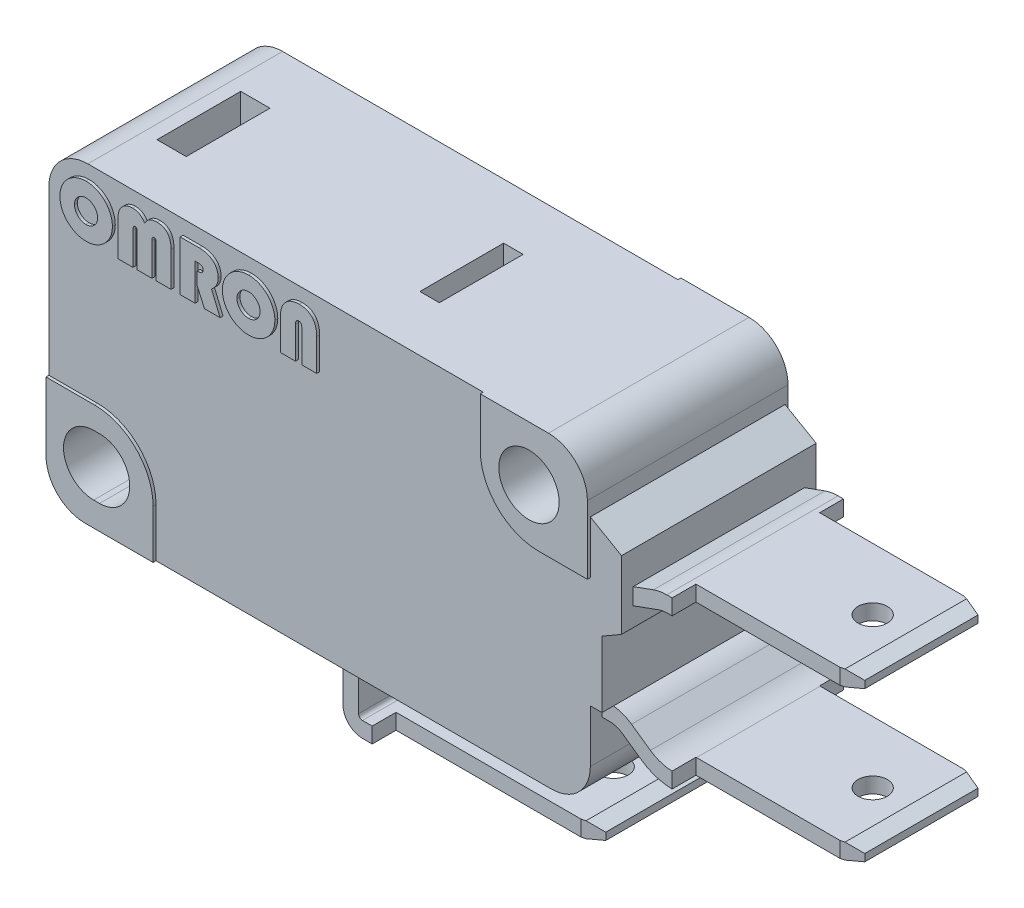
from build123d import *
from OCP.BRepFilletAPI import BRepFilletAPI_MakeChamfer

# Parameters (mm, degrees)
EXTRUDE_1_DEPTH     = 5
EXTRUDE_START       = 0.15
EXTRUDE_2_DEPTH     = 0.15
SKETCH_3_R          = 1.55
CUT_EXTRUDE_1_DEPTH = 21.237156421
CUT_EXTRUDE_2_DEPTH = 2.15
SKETCH_8_R          = 0.5
CUT_EXTRUDE_3_DEPTH = 3
EXTRUDE_3_DEPTH     = 4.4
SKETCH_10_R         = 0.75
SKETCH_10_W         = 8.4
SKETCH_10_H         = 1.225
CUT_EXTRUDE_4_DEPTH = 30.982870109
SKETCH_11_R         = 0.75
SKETCH_11_W         = 10.5
SKETCH_11_H         = 1.225
CUT_EXTRUDE_5_DEPTH = 1
CHAMFER_1_SIZE      = 0.8
CHAMFER_1_SIZE2     = 0.214359354
CHAMFER_2_SIZE      = 0.8
CHAMFER_2_SIZE2     = 0.214359354
CHAMFER_3_SIZE      = 1
CHAMFER_3_SIZE2     = 0.267949192
CHAMFER_4_SIZE      = 1
CHAMFER_4_SIZE2     = 0.267949192
EXTRUDE_6_DEPTH     = 0.15


with BuildPart() as part:
    # 草图1 → 凸台-拉伸1 (new, symmetric)
    with BuildSketch(Plane.XY):
        with BuildLine():
            Line((13.9, -3.25), (14.5, -3.25))
            Line((14.5, -3.25), (14.5, 0.1488893))
            Line((14.5, 0.1488893), (15.5, 0.726239569))
            Line((15.5, 0.726239569), (15.5, 4.226239569))
            Line((15.5, 4.226239569), (13.9, 5.15))
            Line((13.9, 5.15), (13.9, 5.95))
            ThreePointArc((13.9, 5.95), (13.314213562, 7.364213562), (11.9, 7.95))
            Line((11.9, 7.95), (-11.9, 7.95))
            ThreePointArc((-11.9, 7.95), (-13.314213562, 7.364213562), (-13.9, 5.95))
            Line((-13.9, 5.95), (-13.9, -5.95))
            ThreePointArc((-13.9, -5.95), (-13.314213562, -7.364213562), (-11.9, -7.95))
            Line((-11.9, -7.95), (11.9, -7.95))
            ThreePointArc((11.9, -7.95), (13.314213562, -7.364213562), (13.9, -5.95))
            Line((13.9, -5.95), (13.9, -3.25))
        make_face()
    extrude(amount=EXTRUDE_1_DEPTH, both=True)

    # 草图2 → 凸台-拉伸2 (add)
    with BuildSketch(Plane.XY.offset(5).offset(EXTRUDE_START)):
        with BuildLine():
            Line((-13.9, -2.45), (-11.4, -2.45))
            ThreePointArc((-11.4, -2.45), (-9.278679656, -3.328679656), (-8.4, -5.45))
            Line((-8.4, -5.45), (-8.4, -7.95))
            Line((-8.4, -7.95), (-11.9, -7.95))
            ThreePointArc((-11.9, -7.95), (-13.314213562, -7.364213562), (-13.9, -5.95))
            Line((-13.9, -5.95), (-13.9, -2.45))
        make_face()
        with BuildLine():
            Line((8.4, 7.95), (8.4, 5.45))
            ThreePointArc((8.4, 5.45), (9.278679656, 3.328679656), (11.4, 2.45))
            Line((11.4, 2.45), (13.9, 2.45))
            Line((13.9, 2.45), (13.9, 5.15))
            Line((13.9, 5.15), (13.9, 5.95))
            ThreePointArc((13.9, 5.95), (13.314213562, 7.364213562), (11.9, 7.95))
            Line((11.9, 7.95), (8.4, 7.95))
        make_face()
    extrude_2 = extrude(amount=-EXTRUDE_2_DEPTH)

    # 镜向1: 凸台-拉伸2 across plane
    add(extrude_2.mirror(Plane.XY))

    # 草图3 → 切除-拉伸1 (cut, through all)
    with BuildSketch(Plane.XY.offset(5.15)):
        with Locations((10.9, 5.15)):
            Circle(SKETCH_3_R)
        with BuildLine():
            Line((-11.45, -3.6), (-11.15, -3.6))
            ThreePointArc((-11.15, -3.6), (-9.6, -5.15), (-11.15, -6.7))
            Line((-11.15, -6.7), (-11.45, -6.7))
            ThreePointArc((-11.45, -6.7), (-13, -5.15), (-11.45, -3.6))
        make_face()
    extrude(amount=-CUT_EXTRUDE_1_DEPTH, mode=Mode.SUBTRACT)

    # 草图5 → 切除-拉伸2 (cut, symmetric)
    with BuildSketch(Plane.XY):
        with BuildLine():
            Line((-11.2, 7.95), (-9.7, 7.95))
            Line((-9.7, 7.95), (-9.7, 3.45))
            ThreePointArc((-9.7, 3.45), (-10.45, 2.7), (-11.2, 3.45))
            Line((-11.2, 3.45), (-11.2, 7.95))
        make_face()
        with BuildLine():
            Line((2.3, 7.95), (3.3, 7.95))
            Line((3.3, 7.95), (3.3, 6.05))
            ThreePointArc((3.3, 6.05), (2.8, 5.55), (2.3, 6.05))
            Line((2.3, 6.05), (2.3, 7.95))
        make_face()
    extrude(amount=CUT_EXTRUDE_2_DEPTH, both=True, mode=Mode.SUBTRACT)

    # 草图8 → 切除-拉伸3 (cut, symmetric)
    with BuildSketch(Plane.XY):
        with Locations((2.8, 6.05)):
            Circle(SKETCH_8_R)
    extrude(amount=CUT_EXTRUDE_3_DEPTH, both=True, mode=Mode.SUBTRACT)

    # 草图9 → 凸台-拉伸3 (add, symmetric)
    with BuildSketch(Plane.XY):
        with BuildLine():
            Line((0.6, -7.95), (0.6, -10.15))
            ThreePointArc((0.6, -10.15), (0.892893219, -10.857106781), (1.6, -11.15))
            Line((1.6, -11.15), (12.6, -11.15))
            Line((12.6, -11.15), (12.6, -10.35))
            Line((12.6, -10.35), (1.6, -10.35))
            ThreePointArc((1.6, -10.35), (1.458578644, -10.291421356), (1.4, -10.15))
            Line((1.4, -10.15), (1.4, -7.95))
            Line((1.4, -7.95), (0.6, -7.95))
        make_face()
        with BuildLine():
            Line((13.9, -3.25), (14.269402422, -3.25))
            ThreePointArc((14.269402422, -3.25), (14.870814021, -3.342566099), (15.416555295, -3.611695911))
            Line((15.416555295, -3.611695911), (16.382851914, -4.288304089))
            ThreePointArc((16.382851914, -4.288304089), (16.928593188, -4.557433901), (17.530004787, -4.65))
            Line((17.530004787, -4.65), (25.9, -4.65))
            Line((25.9, -4.65), (25.9, -5.45))
            Line((25.9, -5.45), (17.530004787, -5.45))
            ThreePointArc((17.530004787, -5.45), (16.688028549, -5.320407462), (15.923990765, -4.943625724))
            Line((15.923990765, -4.943625724), (14.957694146, -4.267017547))
            ThreePointArc((14.957694146, -4.267017547), (14.630249382, -4.105539659), (14.269402422, -4.05))
            Line((14.269402422, -4.05), (13.9, -4.05))
            Line((13.9, -4.05), (13.9, -3.25))
        make_face()
        with BuildLine():
            Line((15.5, 2.55), (16.542352384, 2.929385242))
            ThreePointArc((16.542352384, 2.929385242), (16.879096316, 3.019615506), (17.226392671, 3.05))
            Line((17.226392671, 3.05), (25.9, 3.05))
            Line((25.9, 3.05), (25.9, 2.25))
            Line((25.9, 2.25), (17.226392671, 2.25))
            ThreePointArc((17.226392671, 2.25), (17.018014858, 2.231769304), (16.815968499, 2.177631145))
            Line((16.815968499, 2.177631145), (15.5, 1.698657782))
            Line((15.5, 1.698657782), (15.5, 2.55))
        make_face()
    extrude(amount=EXTRUDE_3_DEPTH, both=True)

    # 草图10 → 切除-拉伸4 (cut, through all)
    with BuildSketch(Plane(origin=(0, 3.05, 0), x_dir=(1, 0, 0), z_dir=(0, 1, 0))):
        with Locations(Location((23.4, 0, 0), (0, 0, 180))):
            Circle(SKETCH_10_R)
        with Locations((21.7, 3.7875)):
            Rectangle(SKETCH_10_W, SKETCH_10_H)
        with Locations((21.7, -3.7875)):
            Rectangle(SKETCH_10_W, SKETCH_10_H)
    extrude(amount=-CUT_EXTRUDE_4_DEPTH, mode=Mode.SUBTRACT)

    # 草图11 → 切除-拉伸5 (cut)
    with BuildSketch(Plane.XZ.offset(11.15)):
        with Locations(Location((10.1, 0, 0), (0, 0, 270))):
            Circle(SKETCH_11_R)
        with Locations((7.35, 3.7875)):
            Rectangle(SKETCH_11_W, SKETCH_11_H)
        with Locations((7.35, -3.7875)):
            Rectangle(SKETCH_11_W, SKETCH_11_H)
    extrude(amount=-CUT_EXTRUDE_5_DEPTH, mode=Mode.SUBTRACT)

    # 倒角1: one chamfer whose edges measure the first distance from different faces: ONE call of the kernel's chamfer builder (chamfer() names one face for all edges)
    chamfer_1_edges_1 = [part.edges().sort_by_distance(p)[0] for p in [
        (25.9, 3.05, 0),
    ]]
    chamfer_1_side_1 = [part.faces().sort_by_distance(p)[0] for p in [
        (21.450909337, 3.05, 0),
    ]]
    chamfer_1_edges_2 = [part.edges().sort_by_distance(p)[0] for p in [
        (25.9, -4.65, 0),
    ]]
    chamfer_1_side_2 = [part.faces().sort_by_distance(p)[0] for p in [
        (21.657051792, -4.65, 0),
    ]]
    chamfer_1_edges_3 = [part.edges().sort_by_distance(p)[0] for p in [
        (12.6, -10.35, 0),
    ]]
    chamfer_1_side_3 = [part.faces().sort_by_distance(p)[0] for p in [
        (6.930716334, -10.35, 0),
    ]]
    chamfer_1 = BRepFilletAPI_MakeChamfer(part.part.solid().wrapped)
    for e in chamfer_1_edges_1:
        chamfer_1.Add(CHAMFER_1_SIZE, CHAMFER_1_SIZE2, e.wrapped, chamfer_1_side_1[0].wrapped)  # the first distance lies on this face
    for e in chamfer_1_edges_2:
        chamfer_1.Add(CHAMFER_1_SIZE, CHAMFER_1_SIZE2, e.wrapped, chamfer_1_side_2[0].wrapped)  # the first distance lies on this face
    for e in chamfer_1_edges_3:
        chamfer_1.Add(CHAMFER_1_SIZE, CHAMFER_1_SIZE2, e.wrapped, chamfer_1_side_3[0].wrapped)  # the first distance lies on this face
    add(Compound.cast(chamfer_1.Shape()), mode=Mode.REPLACE)

    # 倒角2: one chamfer whose edges measure the first distance from different faces: ONE call of the kernel's chamfer builder (chamfer() names one face for all edges)
    chamfer_2_edges_1 = [part.edges().sort_by_distance(p)[0] for p in [
        (25.9, 2.25, 0),
    ]]
    chamfer_2_side_1 = [part.faces().sort_by_distance(p)[0] for p in [
        (21.450909337, 2.25, 0),
    ]]
    chamfer_2_edges_2 = [part.edges().sort_by_distance(p)[0] for p in [
        (25.9, -5.45, 0),
    ]]
    chamfer_2_side_2 = [part.faces().sort_by_distance(p)[0] for p in [
        (21.657051792, -5.45, 0),
    ]]
    chamfer_2_edges_3 = [part.edges().sort_by_distance(p)[0] for p in [
        (12.6, -11.15, 0),
    ]]
    chamfer_2_side_3 = [part.faces().sort_by_distance(p)[0] for p in [
        (6.930716334, -11.15, 0),
    ]]
    chamfer_2 = BRepFilletAPI_MakeChamfer(part.part.solid().wrapped)
    for e in chamfer_2_edges_1:
        chamfer_2.Add(CHAMFER_2_SIZE, CHAMFER_2_SIZE2, e.wrapped, chamfer_2_side_1[0].wrapped)  # the first distance lies on this face
    for e in chamfer_2_edges_2:
        chamfer_2.Add(CHAMFER_2_SIZE, CHAMFER_2_SIZE2, e.wrapped, chamfer_2_side_2[0].wrapped)  # the first distance lies on this face
    for e in chamfer_2_edges_3:
        chamfer_2.Add(CHAMFER_2_SIZE, CHAMFER_2_SIZE2, e.wrapped, chamfer_2_side_3[0].wrapped)  # the first distance lies on this face
    add(Compound.cast(chamfer_2.Shape()), mode=Mode.REPLACE)

    # 倒角3: one chamfer whose edges measure the first distance from different faces: ONE call of the kernel's chamfer builder (chamfer() names one face for all edges)
    chamfer_3_edges_1 = [part.edges().sort_by_distance(p)[0] for p in [
        (25.9, -5.05, -3.175),
    ]]
    chamfer_3_side_1 = [part.faces().sort_by_distance(p)[0] for p in [
        (21.596996446, -5.049999764, -3.175),
    ]]
    chamfer_3_edges_2 = [part.edges().sort_by_distance(p)[0] for p in [
        (25.9, 2.65, -3.175),
    ]]
    chamfer_3_side_2 = [part.faces().sort_by_distance(p)[0] for p in [
        (21.596996847, 2.65, -3.175),
    ]]
    chamfer_3_edges_3 = [part.edges().sort_by_distance(p)[0] for p in [
        (12.6, -10.75, -3.175),
    ]]
    chamfer_3_side_3 = [part.faces().sort_by_distance(p)[0] for p in [
        (7.246144134, -10.75, -3.175),
    ]]
    chamfer_3 = BRepFilletAPI_MakeChamfer(part.part.solid().wrapped)
    for e in chamfer_3_edges_1:
        chamfer_3.Add(CHAMFER_3_SIZE, CHAMFER_3_SIZE2, e.wrapped, chamfer_3_side_1[0].wrapped)  # the first distance lies on this face
    for e in chamfer_3_edges_2:
        chamfer_3.Add(CHAMFER_3_SIZE, CHAMFER_3_SIZE2, e.wrapped, chamfer_3_side_2[0].wrapped)  # the first distance lies on this face
    for e in chamfer_3_edges_3:
        chamfer_3.Add(CHAMFER_3_SIZE, CHAMFER_3_SIZE2, e.wrapped, chamfer_3_side_3[0].wrapped)  # the first distance lies on this face
    add(Compound.cast(chamfer_3.Shape()), mode=Mode.REPLACE)

    # 倒角4: one chamfer whose edges measure the first distance from different faces: ONE call of the kernel's chamfer builder (chamfer() names one face for all edges)
    chamfer_4_edges_1 = [part.edges().sort_by_distance(p)[0] for p in [
        (25.9, -5.05, 3.175),
    ]]
    chamfer_4_side_1 = [part.faces().sort_by_distance(p)[0] for p in [
        (21.596996446, -5.049999764, 3.175),
    ]]
    chamfer_4_edges_2 = [part.edges().sort_by_distance(p)[0] for p in [
        (25.9, 2.65, 3.175),
    ]]
    chamfer_4_side_2 = [part.faces().sort_by_distance(p)[0] for p in [
        (21.596996847, 2.65, 3.175),
    ]]
    chamfer_4_edges_3 = [part.edges().sort_by_distance(p)[0] for p in [
        (12.6, -10.75, 3.175),
    ]]
    chamfer_4_side_3 = [part.faces().sort_by_distance(p)[0] for p in [
        (7.246144134, -10.75, 3.175),
    ]]
    chamfer_4 = BRepFilletAPI_MakeChamfer(part.part.solid().wrapped)
    for e in chamfer_4_edges_1:
        chamfer_4.Add(CHAMFER_4_SIZE, CHAMFER_4_SIZE2, e.wrapped, chamfer_4_side_1[0].wrapped)  # the first distance lies on this face
    for e in chamfer_4_edges_2:
        chamfer_4.Add(CHAMFER_4_SIZE, CHAMFER_4_SIZE2, e.wrapped, chamfer_4_side_2[0].wrapped)  # the first distance lies on this face
    for e in chamfer_4_edges_3:
        chamfer_4.Add(CHAMFER_4_SIZE, CHAMFER_4_SIZE2, e.wrapped, chamfer_4_side_3[0].wrapped)  # the first distance lies on this face
    add(Compound.cast(chamfer_4.Shape()), mode=Mode.REPLACE)

    # 草图12 → 凸台-拉伸6 (add)
    # profile 1 of 5: a face of its own
    with BuildSketch(Plane.XY.offset(5)):
        with BuildLine():
            add(Edge.make_bspline(
                [(-11.839991798, 7.284851975), (-11.810073224, 7.284327276), (-11.750675759, 7.283285589), (-11.662283846, 7.274595125), (-11.575549668, 7.260812561), (-11.490214484, 7.241324627), (-11.406864613, 7.215353494), (-11.324502331, 7.185023297), (-11.244436385, 7.1478037), (-11.165899619, 7.106345186), (-11.090511472, 7.059561807), (-11.018297745, 7.008864953), (-10.950378811, 6.95373237), (-10.886701297, 6.894389736), (-10.826790936, 6.831277485), (-10.771135463, 6.763895002), (-10.719655155, 6.692187959), (-10.672730505, 6.616922671), (-10.630327479, 6.539049624), (-10.593456274, 6.45921368), (-10.562226952, 6.377688868), (-10.536396609, 6.294753684), (-10.517163106, 6.210101031), (-10.502331332, 6.124247216), (-10.493964618, 6.036701875), (-10.492870367, 5.977867341), (-10.492320887, 5.948323445)],
                knots=[0, 0, 0, 0, 1.021661308, 2.028308306, 3.030389079, 4.019702427, 5.014833943, 6.01032923, 7.015036116, 8.027997564, 9.041872037, 10.04316966, 11.039694905, 12.027034081, 13.014087999, 14.009724715, 15.009534675, 16.026756487, 17.037133186, 18.036077674, 19.027888702, 20.016958036, 21.000091493, 21.990684927, 22.991017831, 24, 24, 24, 24], degree=3))
            add(Edge.make_bspline(
                [(-10.492320887, 5.948323445), (-10.492870761, 5.918779673), (-10.493965794, 5.859945386), (-10.502326694, 5.772398208), (-10.517180262, 5.686551281), (-10.536293747, 5.602046231), (-10.562352659, 5.519370522), (-10.593412015, 5.437969296), (-10.630511869, 5.358069672), (-10.672390966, 5.279897616), (-10.719854097, 5.204951969), (-10.771116293, 5.133302457), (-10.826761684, 5.065889776), (-10.886923526, 5.002874533), (-10.949968186, 4.942805024), (-11.018701336, 4.888496279), (-11.090282184, 4.836947876), (-11.165961989, 4.790412657), (-11.244257983, 4.748631429), (-11.324795915, 4.71252768), (-11.406606692, 4.680921455), (-11.490346315, 4.656110733), (-11.575528182, 4.636325447), (-11.662289633, 4.62262666), (-11.750674285, 4.613913889), (-11.81007273, 4.612875215), (-11.839991798, 4.612352033)],
                knots=[0, 0, 0, 0, 1.009153083, 2.009655437, 3.000416671, 3.983716664, 4.96689387, 5.958872904, 6.957986607, 7.974114181, 8.986134409, 9.986113729, 10.9819191, 11.969140218, 12.960977253, 13.95368625, 14.958823603, 15.972869819, 16.986002856, 17.988253375, 18.986157985, 19.979616663, 20.969097594, 21.971348113, 22.978165629, 24, 24, 24, 24], degree=3))
            add(Edge.make_bspline(
                [(-11.839991798, 4.612352033), (-11.869910881, 4.61287518), (-11.929309358, 4.613913786), (-12.017693781, 4.622627065), (-12.104456089, 4.636323945), (-12.189634791, 4.656116272), (-12.273386259, 4.68090064), (-12.355310552, 4.712667156), (-12.436166343, 4.748477792), (-12.514569817, 4.790432512), (-12.590260895, 4.836942604), (-12.661838761, 4.888497665), (-12.730572677, 4.942804661), (-12.793617211, 5.002874606), (-12.853778795, 5.065889843), (-12.909425354, 5.133302108), (-12.960683095, 5.204953308), (-13.008163097, 5.279892539), (-13.049979178, 5.358088563), (-13.087282054, 5.437840502), (-13.117475547, 5.519500144), (-13.143736666, 5.602028431), (-13.162790692, 5.686556088), (-13.177660321, 5.772396908), (-13.186016936, 5.859945716), (-13.187112546, 5.918779783), (-13.187662709, 5.948323445)],
                knots=[0, 0, 0, 0, 1.021684044, 2.028353444, 3.030456519, 4.019791883, 5.013104409, 6.010862213, 7.018749798, 8.031733789, 9.045630825, 10.050620308, 11.043183264, 12.034874386, 13.02195027, 14.017609144, 15.017441353, 16.029312699, 17.045290786, 18.044257506, 19.033836829, 20.016869396, 21.000024732, 21.990640211, 22.990995377, 24, 24, 24, 24], degree=3))
            add(Edge.make_bspline(
                [(-13.187662709, 5.948323445), (-13.187112939, 5.977867231), (-13.186018112, 6.036701546), (-13.177655681, 6.124248515), (-13.162807851, 6.210096225), (-13.143633913, 6.294771527), (-13.117599886, 6.377558735), (-13.087237778, 6.45934248), (-13.050163925, 6.53903087), (-13.007823594, 6.61692776), (-12.960882032, 6.692186619), (-12.909406184, 6.76389535), (-12.853749543, 6.831277418), (-12.793839438, 6.894389662), (-12.730162056, 6.953732737), (-12.662242332, 7.008863545), (-12.590031666, 7.059567124), (-12.514631925, 7.106325077), (-12.435989008, 7.147957464), (-12.355603598, 7.184885152), (-12.273128647, 7.215374716), (-12.189766541, 7.241318981), (-12.104434625, 7.260814091), (-12.017699562, 7.274594713), (-11.929307885, 7.283285694), (-11.869910388, 7.284327311), (-11.839991798, 7.284851975)],
                knots=[0, 0, 0, 0, 1.00883439, 2.009020783, 2.999469132, 3.982458596, 4.971383068, 5.960795436, 6.959593616, 7.969822333, 8.98689516, 9.986558684, 10.982049577, 11.968958928, 12.956153496, 13.952532787, 14.953683757, 15.967409735, 16.980222822, 17.99055106, 18.985900543, 19.98088631, 20.97005476, 21.971988766, 22.978488327, 24, 24, 24, 24], degree=3))
        make_face()
        with BuildLine():
            add(Edge.make_bspline(
                [(-11.843891631, 5.35944864), (-11.823816343, 5.360043883), (-11.784071756, 5.361222332), (-11.725518417, 5.368774544), (-11.669474516, 5.383075873), (-11.615765049, 5.40207715), (-11.563924484, 5.425952438), (-11.515020492, 5.456468843), (-11.467842494, 5.491658767), (-11.423744945, 5.532083862), (-11.383525093, 5.576133779), (-11.347943814, 5.622839772), (-11.317796046, 5.671604795), (-11.293723612, 5.722956508), (-11.274747747, 5.77613103), (-11.260505509, 5.831437776), (-11.252853781, 5.889239011), (-11.25170169, 5.928432438), (-11.251116993, 5.948323445)],
                knots=[0, 0, 0, 0, 1.037369248, 2.053759453, 3.042788757, 4.01997185, 4.994371679, 5.985028633, 6.992502963, 8.031645644, 9.070788326, 10.070603235, 11.061260189, 12.026976158, 12.995120048, 13.974843604, 14.972215384, 16, 16, 16, 16], degree=3))
            add(Edge.make_bspline(
                [(-11.251116993, 5.948323445), (-11.251614097, 5.968229317), (-11.252594243, 6.007477938), (-11.261533408, 6.065225549), (-11.274408552, 6.121260415), (-11.294245, 6.174676566), (-11.31895887, 6.226044923), (-11.349348226, 6.275199911), (-11.384816155, 6.322702568), (-11.426187787, 6.366584455), (-11.470069664, 6.40795582), (-11.5175721, 6.44342477), (-11.566727945, 6.473810454), (-11.618093157, 6.498537721), (-11.671351474, 6.518260907), (-11.727155856, 6.53131824), (-11.784740379, 6.540164447), (-11.82398685, 6.541153553), (-11.843891631, 6.541655202)],
                knots=[0, 0, 0, 0, 1.025725638, 2.022434234, 3.007203552, 3.985667517, 4.953578649, 5.942251004, 6.961114924, 8.0046544, 9.048193875, 10.067057795, 11.05573015, 12.023641282, 13.002105247, 13.977565766, 14.974274362, 16, 16, 16, 16], degree=3))
            add(Edge.make_bspline(
                [(-11.843891631, 6.541655202), (-11.86379772, 6.541158584), (-11.903046768, 6.540179396), (-11.960791258, 6.53123323), (-12.016837752, 6.518384167), (-12.070368114, 6.498392746), (-12.122038945, 6.473945443), (-12.17128493, 6.443603613), (-12.218333824, 6.407586087), (-12.262688797, 6.36678028), (-12.304114535, 6.322854765), (-12.338933997, 6.275020764), (-12.369411721, 6.22606679), (-12.394087265, 6.17467069), (-12.413934029, 6.121262007), (-12.426806378, 6.065225118), (-12.435746293, 6.00747805), (-12.436726336, 5.968229355), (-12.437223388, 5.948323445)],
                knots=[0, 0, 0, 0, 1.024980994, 2.020966011, 3.005020418, 3.982774049, 4.958606057, 5.946560666, 6.957057065, 8.006883537, 9.049665437, 10.062062882, 11.050017492, 12.017225951, 12.994979582, 13.979033989, 14.975019006, 16, 16, 16, 16], degree=3))
            add(Edge.make_bspline(
                [(-12.437223388, 5.948323445), (-12.436638692, 5.928432438), (-12.435486601, 5.889239011), (-12.427834872, 5.831437776), (-12.413592635, 5.776131028), (-12.394616766, 5.722956515), (-12.370544348, 5.671604768), (-12.34039652, 5.622839874), (-12.304815469, 5.576133388), (-12.264594735, 5.532085384), (-12.220500468, 5.491653169), (-12.173310652, 5.456488886), (-12.124306511, 5.425789862), (-12.072138947, 5.402215876), (-12.018319076, 5.383053554), (-11.962261993, 5.368780707), (-11.903712244, 5.361220736), (-11.863967167, 5.360043348), (-11.843891631, 5.35944864)],
                knots=[0, 0, 0, 0, 1.027226011, 2.024055714, 3.003246787, 3.970864486, 4.936055584, 5.926174111, 6.925445617, 7.964023519, 9.002601422, 10.009528185, 10.999646713, 11.982213023, 12.958865012, 13.947356774, 14.963194567, 16, 16, 16, 16], degree=3))
        make_face(mode=Mode.SUBTRACT)
    # profile 2 of 5: a face of its own
    with BuildSketch(Plane.XY.offset(5)):
        with BuildLine():
            Line((-10.199833401, 4.654693079), (-10.199833401, 6.507113822))
            add(Edge.make_bspline(
                [(-10.199833401, 6.507113822), (-10.199238422, 6.535004889), (-10.19807221, 6.589673842), (-10.187517826, 6.669762946), (-10.171836884, 6.746165648), (-10.148794096, 6.818580558), (-10.119173777, 6.886932172), (-10.082787005, 6.951382185), (-10.039586228, 7.011665795), (-9.990645064, 7.067944512), (-9.936573418, 7.118795455), (-9.87813828, 7.16326071), (-9.815943005, 7.20080454), (-9.749816998, 7.231590689), (-9.679773702, 7.255578142), (-9.606084879, 7.272856225), (-9.528603921, 7.283007754), (-9.475794682, 7.28422871), (-9.448836962, 7.284851975)],
                knots=[0, 0, 0, 0, 1.102663291, 2.161317456, 3.189909821, 4.184149151, 5.161173166, 6.13146464, 7.105723695, 8.089680947, 9.077004599, 10.036307647, 10.9886396, 11.944900811, 12.915859305, 13.911806509, 14.934032427, 16, 16, 16, 16], degree=3))
            add(Edge.make_bspline(
                [(-9.448836962, 7.284851975), (-9.416618779, 7.283914898), (-9.353734749, 7.282085893), (-9.262632689, 7.263903062), (-9.17690412, 7.236352199), (-9.097031368, 7.196398955), (-9.023432705, 7.144351472), (-8.95571787, 7.081214142), (-8.893172709, 7.007369039), (-8.858343365, 6.951437988), (-8.840462991, 6.922724612)],
                knots=[0, 0, 0, 0, 1.037369451, 2.024756404, 2.982649248, 3.933049122, 4.891334709, 5.878358653, 6.910810976, 8, 8, 8, 8], degree=3))
            add(Edge.make_bspline(
                [(-8.840462991, 6.922724612), (-8.821065782, 6.952539658), (-8.783628759, 7.010083327), (-8.718469493, 7.086078868), (-8.648561866, 7.148949243), (-8.573554847, 7.200173438), (-8.491188448, 7.238270959), (-8.400897054, 7.265759021), (-8.301737773, 7.281758752), (-8.232705063, 7.283797312), (-8.196990522, 7.284851975)],
                knots=[0, 0, 0, 0, 1.097134874, 2.117493542, 3.079635451, 3.992275589, 4.910372732, 5.869641242, 6.897844434, 8, 8, 8, 8], degree=3))
            add(Edge.make_bspline(
                [(-8.196990522, 7.284851975), (-8.168919377, 7.284235317), (-8.114259941, 7.283034574), (-8.034723952, 7.272990171), (-7.960396511, 7.255842073), (-7.891149015, 7.231620814), (-7.82679159, 7.201211791), (-7.767775075, 7.16322197), (-7.713165151, 7.119317205), (-7.664862413, 7.067387177), (-7.621020871, 7.010024136), (-7.583693985, 6.94584389), (-7.552063447, 6.875956796), (-7.525558304, 6.800166437), (-7.505900306, 6.717975024), (-7.491636394, 6.629893059), (-7.482389586, 6.5357228), (-7.48153416, 6.470923836), (-7.481092581, 6.437473945)],
                knots=[0, 0, 0, 0, 1.066598017, 2.076853064, 3.040727948, 3.960382046, 4.860103194, 5.73921303, 6.622167718, 7.515861307, 8.427763883, 9.361048407, 10.330694431, 11.33961724, 12.407802041, 13.537962884, 14.72907115, 16, 16, 16, 16], degree=3))
            Line((-7.481092581, 6.437473945), (-7.481092581, 4.654693079))
            Line((-7.481092581, 4.654693079), (-8.247131234, 4.654693079))
            Line((-8.247131234, 4.654693079), (-8.247131234, 6.326050141))
            add(Edge.make_bspline(
                [(-8.247131234, 6.326050141), (-8.247250471, 6.343329859), (-8.247470091, 6.375157126), (-8.251296244, 6.418738159), (-8.257206105, 6.454219499), (-8.264998956, 6.482392649), (-8.277012757, 6.504351653), (-8.294788532, 6.519549951), (-8.317622192, 6.52885694), (-8.334502661, 6.529573324), (-8.343512825, 6.529955702)],
                knots=[0, 0, 0, 0, 1.623684708, 2.990641638, 4.106939268, 5.001409125, 5.728884434, 6.421825748, 7.157629609, 8, 8, 8, 8], degree=3))
            add(Edge.make_bspline(
                [(-8.343512825, 6.529955702), (-8.352716482, 6.529588781), (-8.370386749, 6.528884323), (-8.394628553, 6.518737073), (-8.414840674, 6.503056471), (-8.431504982, 6.481464613), (-8.444001864, 6.453803192), (-8.452598283, 6.420257693), (-8.458221505, 6.38102107), (-8.458622368, 6.352814337), (-8.458836462, 6.33774964)],
                knots=[0, 0, 0, 0, 0.870208494, 1.670728877, 2.451709394, 3.282275218, 4.238613916, 5.318652993, 6.56794201, 8, 8, 8, 8], degree=3))
            Line((-8.458836462, 6.33774964), (-8.458836462, 4.654693079))
            Line((-8.458836462, 4.654693079), (-9.221532401, 4.654693079))
            Line((-9.221532401, 4.654693079), (-9.221532401, 6.326050141))
            add(Edge.make_bspline(
                [(-9.221532401, 6.326050141), (-9.221651038, 6.342773209), (-9.221870255, 6.373674252), (-9.225758459, 6.416320921), (-9.231692732, 6.451595646), (-9.239444844, 6.480389514), (-9.251826208, 6.50316279), (-9.270403356, 6.519100776), (-9.294361722, 6.529036497), (-9.312235735, 6.52963499), (-9.321813825, 6.529955702)],
                knots=[0, 0, 0, 0, 1.554968012, 2.873284574, 3.977956704, 4.879642019, 5.638089054, 6.348181832, 7.114845454, 8, 8, 8, 8], degree=3))
            add(Edge.make_bspline(
                [(-9.321813825, 6.529955702), (-9.330655607, 6.529367056), (-9.347607888, 6.528238448), (-9.371053683, 6.51789693), (-9.39131704, 6.5019435), (-9.406903874, 6.478412297), (-9.419084005, 6.449115876), (-9.426774177, 6.41344544), (-9.432702268, 6.371929501), (-9.433050946, 6.342048476), (-9.433237629, 6.326050141)],
                knots=[0, 0, 0, 0, 0.812646849, 1.558081647, 2.326829032, 3.164255741, 4.132651413, 5.243379863, 6.524102441, 8, 8, 8, 8], degree=3))
            Line((-9.433237629, 6.326050141), (-9.433237629, 4.654693079))
            Line((-9.433237629, 4.654693079), (-10.199833401, 4.654693079))
        make_face()
    # profile 3 of 5: a face of its own
    with BuildSketch(Plane.XY.offset(5)):
        with BuildLine():
            Line((-6.245402593, 6.529955702), (-6.245402593, 4.654693079))
            Line((-6.245402593, 4.654693079), (-7.008098532, 4.654693079))
            Line((-7.008098532, 4.654693079), (-7.008098532, 7.223011764))
            Line((-7.008098532, 7.223011764), (-6.029797532, 7.223011764))
            add(Edge.make_bspline(
                [(-6.029797532, 7.223011764), (-5.993184145, 7.222261302), (-5.921824432, 7.220798648), (-5.817875425, 7.209493673), (-5.719861379, 7.191188398), (-5.627557429, 7.165848091), (-5.541374844, 7.132277188), (-5.461170845, 7.091327811), (-5.386490918, 7.043443953), (-5.318923955, 6.987632711), (-5.257847466, 6.926389158), (-5.205057527, 6.85978581), (-5.159014627, 6.789391044), (-5.123176891, 6.713564327), (-5.094335602, 6.633770947), (-5.07386895, 6.549368718), (-5.061294341, 6.460324949), (-5.059971173, 6.399446499), (-5.059296198, 6.368391186)],
                knots=[0, 0, 0, 0, 1.205518528, 2.349562907, 3.438641392, 4.486182617, 5.496929055, 6.478808746, 7.447400395, 8.412103695, 9.359141492, 10.290349245, 11.20639267, 12.122701433, 13.045416251, 13.996178639, 14.977810715, 16, 16, 16, 16], degree=3))
            add(Edge.make_bspline(
                [(-5.059296198, 6.368391186), (-5.06044182, 6.336208837), (-5.06269386, 6.272945407), (-5.078292373, 6.179910158), (-5.106102258, 6.091663845), (-5.143493353, 6.006998913), (-5.192703932, 5.927215725), (-5.251602615, 5.850591662), (-5.322007368, 5.77870919), (-5.375282601, 5.735722554), (-5.402481515, 5.713776337)],
                knots=[0, 0, 0, 0, 1.006052783, 1.977678795, 2.938069743, 3.891839897, 4.863622002, 5.861128799, 6.908029685, 8, 8, 8, 8], degree=3))
            Line((-5.402481515, 5.713776337), (-4.959571894, 4.654693079))
            Line((-4.959571894, 4.654693079), (-5.76405176, 4.654693079))
            Line((-5.76405176, 4.654693079), (-6.133978789, 5.482571944))
            Line((-6.133978789, 5.482571944), (-6.133978789, 6.141086626))
            Line((-6.133978789, 6.141086626), (-6.072138578, 6.141086626))
            add(Edge.make_bspline(
                [(-6.072138578, 6.141086626), (-6.053152367, 6.141686707), (-6.017511835, 6.142813168), (-5.967592011, 6.152125962), (-5.924910508, 6.16797953), (-5.889714063, 6.191384539), (-5.862265859, 6.22159601), (-5.842876301, 6.258556678), (-5.831879689, 6.301844162), (-5.830511666, 6.332670832), (-5.829791804, 6.348892021)],
                knots=[0, 0, 0, 0, 1.246893405, 2.340643143, 3.321932138, 4.218857632, 5.091461181, 5.975846322, 6.934877491, 8, 8, 8, 8], degree=3))
            add(Edge.make_bspline(
                [(-5.829791804, 6.348892021), (-5.830614098, 6.363101335), (-5.832188454, 6.39030633), (-5.845229387, 6.428760947), (-5.86854753, 6.460695828), (-5.90018688, 6.487148737), (-5.941041681, 6.50609175), (-5.989723495, 6.520788519), (-6.047386319, 6.528519842), (-6.088647499, 6.529457364), (-6.11057979, 6.529955702)],
                knots=[0, 0, 0, 0, 0.901674002, 1.726334911, 2.538321715, 3.38431502, 4.318296618, 5.37836456, 6.60647533, 8, 8, 8, 8], degree=3))
            Line((-6.11057979, 6.529955702), (-6.245402593, 6.529955702))
        make_face()
    # profile 4 of 5: a face of its own
    with BuildSketch(Plane.XY.offset(5)):
        with BuildLine():
            add(Edge.make_bspline(
                [(-3.496577346, 7.284851975), (-3.466658772, 7.284327276), (-3.407261307, 7.283285589), (-3.318869394, 7.274595125), (-3.232135216, 7.260812561), (-3.146800032, 7.241324627), (-3.063450161, 7.215353494), (-2.981087879, 7.185023297), (-2.901021932, 7.1478037), (-2.822485167, 7.106345186), (-2.74709702, 7.059561807), (-2.674883292, 7.008864953), (-2.606964359, 6.95373237), (-2.543286845, 6.894389736), (-2.483376484, 6.831277485), (-2.42772101, 6.763895002), (-2.376240703, 6.692187959), (-2.329316053, 6.616922671), (-2.286913027, 6.539049624), (-2.250041822, 6.45921368), (-2.218812499, 6.377688868), (-2.192982157, 6.294753684), (-2.173748653, 6.210101031), (-2.15891688, 6.124247216), (-2.150550165, 6.036701875), (-2.149455915, 5.977867341), (-2.148906435, 5.948323445)],
                knots=[0, 0, 0, 0, 1.021661308, 2.028308306, 3.030389079, 4.019702427, 5.014833943, 6.01032923, 7.015036116, 8.027997564, 9.041872037, 10.04316966, 11.039694905, 12.027034081, 13.014087999, 14.009724715, 15.009534675, 16.026756487, 17.037133186, 18.036077674, 19.027888702, 20.016958036, 21.000091493, 21.990684927, 22.991017831, 24, 24, 24, 24], degree=3))
            add(Edge.make_bspline(
                [(-2.148906435, 5.948323445), (-2.149456308, 5.918779673), (-2.150551341, 5.859945386), (-2.158912241, 5.772398208), (-2.173765809, 5.686551281), (-2.192879295, 5.602046231), (-2.218938207, 5.519370522), (-2.249997562, 5.437969296), (-2.287097417, 5.358069672), (-2.328976514, 5.279897616), (-2.376439644, 5.204951969), (-2.427701841, 5.133302457), (-2.483347232, 5.065889776), (-2.543509074, 5.002874533), (-2.606553734, 4.942805024), (-2.675286884, 4.888496279), (-2.746867732, 4.836947876), (-2.822547537, 4.790412657), (-2.900843531, 4.748631429), (-2.981381463, 4.71252768), (-3.063192239, 4.680921455), (-3.146931863, 4.656110733), (-3.23211373, 4.636325447), (-3.318875181, 4.62262666), (-3.407259832, 4.613913889), (-3.466658278, 4.612875215), (-3.496577346, 4.612352033)],
                knots=[0, 0, 0, 0, 1.009153083, 2.009655437, 3.000416671, 3.983716664, 4.96689387, 5.958872904, 6.957986607, 7.974114181, 8.986134409, 9.986113729, 10.9819191, 11.969140218, 12.960977253, 13.95368625, 14.958823603, 15.972869819, 16.986002856, 17.988253375, 18.986157985, 19.979616663, 20.969097594, 21.971348113, 22.978165629, 24, 24, 24, 24], degree=3))
            add(Edge.make_bspline(
                [(-3.496577346, 4.612352033), (-3.526496429, 4.61287518), (-3.585894905, 4.613913786), (-3.674279329, 4.622627065), (-3.761041637, 4.636323945), (-3.846220339, 4.656116272), (-3.929971807, 4.68090064), (-4.0118961, 4.712667156), (-4.092751891, 4.748477792), (-4.171155365, 4.790432512), (-4.246846443, 4.836942604), (-4.318424309, 4.888497665), (-4.387158225, 4.942804661), (-4.450202759, 5.002874606), (-4.510364343, 5.065889843), (-4.566010902, 5.133302108), (-4.617268643, 5.204953308), (-4.664748645, 5.279892539), (-4.706564726, 5.358088563), (-4.743867602, 5.437840502), (-4.774061094, 5.519500144), (-4.800322214, 5.602028431), (-4.819376239, 5.686556088), (-4.834245868, 5.772396908), (-4.842602483, 5.859945716), (-4.843698093, 5.918779783), (-4.844248257, 5.948323445)],
                knots=[0, 0, 0, 0, 1.021684044, 2.028353444, 3.030456519, 4.019791883, 5.013104409, 6.010862213, 7.018749798, 8.031733789, 9.045630825, 10.050620308, 11.043183264, 12.034874386, 13.02195027, 14.017609144, 15.017441353, 16.029312699, 17.045290786, 18.044257506, 19.033836829, 20.016869396, 21.000024732, 21.990640211, 22.990995377, 24, 24, 24, 24], degree=3))
            add(Edge.make_bspline(
                [(-4.844248257, 5.948323445), (-4.843698487, 5.977867231), (-4.84260366, 6.036701546), (-4.834241229, 6.124248515), (-4.819393399, 6.210096225), (-4.800219461, 6.294771527), (-4.774185434, 6.377558735), (-4.743823326, 6.45934248), (-4.706749473, 6.53903087), (-4.664409142, 6.61692776), (-4.61746758, 6.692186619), (-4.565991731, 6.76389535), (-4.510335091, 6.831277418), (-4.450424986, 6.894389662), (-4.386747604, 6.953732737), (-4.31882788, 7.008863545), (-4.246617214, 7.059567124), (-4.171217473, 7.106325077), (-4.092574556, 7.147957464), (-4.012189146, 7.184885152), (-3.929714195, 7.215374716), (-3.846352088, 7.241318981), (-3.761020173, 7.260814091), (-3.67428511, 7.274594713), (-3.585893432, 7.283285694), (-3.526495936, 7.284327311), (-3.496577346, 7.284851975)],
                knots=[0, 0, 0, 0, 1.00883439, 2.009020783, 2.999469132, 3.982458596, 4.971383068, 5.960795436, 6.959593616, 7.969822333, 8.98689516, 9.986558684, 10.982049577, 11.968958928, 12.956153496, 13.952532787, 14.953683757, 15.967409735, 16.980222822, 17.99055106, 18.985900543, 19.98088631, 20.97005476, 21.971988766, 22.978488327, 24, 24, 24, 24], degree=3))
        make_face()
        with BuildLine():
            add(Edge.make_bspline(
                [(-3.500477179, 5.35944864), (-3.480401891, 5.360043883), (-3.440657304, 5.361222332), (-3.382103965, 5.368774544), (-3.326060063, 5.383075873), (-3.272350597, 5.40207715), (-3.220510031, 5.425952438), (-3.17160604, 5.456468843), (-3.124428042, 5.491658767), (-3.080330492, 5.532083862), (-3.04011064, 5.576133779), (-3.004529362, 5.622839772), (-2.974381594, 5.671604795), (-2.950309159, 5.722956508), (-2.931333295, 5.77613103), (-2.917091056, 5.831437776), (-2.909439328, 5.889239011), (-2.908287237, 5.928432438), (-2.907702541, 5.948323445)],
                knots=[0, 0, 0, 0, 1.037369248, 2.053759453, 3.042788757, 4.01997185, 4.994371679, 5.985028633, 6.992502963, 8.031645644, 9.070788326, 10.070603235, 11.061260189, 12.026976158, 12.995120048, 13.974843604, 14.972215384, 16, 16, 16, 16], degree=3))
            add(Edge.make_bspline(
                [(-2.907702541, 5.948323445), (-2.908199645, 5.968229317), (-2.90917979, 6.007477938), (-2.918118956, 6.065225549), (-2.930994099, 6.121260415), (-2.950830547, 6.174676566), (-2.975544417, 6.226044923), (-3.005933774, 6.275199911), (-3.041401702, 6.322702568), (-3.082773334, 6.366584455), (-3.126655212, 6.40795582), (-3.174157648, 6.44342477), (-3.223313493, 6.473810454), (-3.274678705, 6.498537721), (-3.327937021, 6.518260907), (-3.383741404, 6.53131824), (-3.441325927, 6.540164447), (-3.480572398, 6.541153553), (-3.500477179, 6.541655202)],
                knots=[0, 0, 0, 0, 1.025725638, 2.022434234, 3.007203552, 3.985667517, 4.953578649, 5.942251004, 6.961114924, 8.0046544, 9.048193875, 10.067057795, 11.05573015, 12.023641282, 13.002105247, 13.977565766, 14.974274362, 16, 16, 16, 16], degree=3))
            add(Edge.make_bspline(
                [(-3.500477179, 6.541655202), (-3.520383268, 6.541158584), (-3.559632316, 6.540179396), (-3.617376806, 6.53123323), (-3.6734233, 6.518384167), (-3.726953662, 6.498392746), (-3.778624493, 6.473945443), (-3.827870478, 6.443603613), (-3.874919372, 6.407586087), (-3.919274345, 6.36678028), (-3.960700083, 6.322854765), (-3.995519545, 6.275020764), (-4.025997268, 6.22606679), (-4.050672813, 6.17467069), (-4.070519576, 6.121262007), (-4.083391926, 6.065225118), (-4.092331841, 6.00747805), (-4.093311884, 5.968229355), (-4.093808936, 5.948323445)],
                knots=[0, 0, 0, 0, 1.024980994, 2.020966011, 3.005020418, 3.982774049, 4.958606057, 5.946560666, 6.957057065, 8.006883537, 9.049665437, 10.062062882, 11.050017492, 12.017225951, 12.994979582, 13.979033989, 14.975019006, 16, 16, 16, 16], degree=3))
            add(Edge.make_bspline(
                [(-4.093808936, 5.948323445), (-4.093224239, 5.928432438), (-4.092072148, 5.889239011), (-4.08442042, 5.831437776), (-4.070178183, 5.776131028), (-4.051202314, 5.722956515), (-4.027129895, 5.671604768), (-3.996982068, 5.622839874), (-3.961401017, 5.576133388), (-3.921180283, 5.532085384), (-3.877086015, 5.491653169), (-3.8298962, 5.456488886), (-3.780892059, 5.425789862), (-3.728724495, 5.402215876), (-3.674904624, 5.383053554), (-3.618847541, 5.368780707), (-3.560297792, 5.361220736), (-3.520552715, 5.360043348), (-3.500477179, 5.35944864)],
                knots=[0, 0, 0, 0, 1.027226011, 2.024055714, 3.003246787, 3.970864486, 4.936055584, 5.926174111, 6.925445617, 7.964023519, 9.002601422, 10.009528185, 10.999646713, 11.982213023, 12.958865012, 13.947356774, 14.963194567, 16, 16, 16, 16], degree=3))
        make_face(mode=Mode.SUBTRACT)
    # profile 5 of 5: a face of its own
    with BuildSketch(Plane.XY.offset(5)):
        with BuildLine():
            Line((-1.856418949, 4.654693079), (-1.856418949, 6.322150308))
            add(Edge.make_bspline(
                [(-1.856418949, 6.322150308), (-1.855742258, 6.35747117), (-1.854416627, 6.42666446), (-1.841922252, 6.527739821), (-1.821430114, 6.62365044), (-1.792404669, 6.714134804), (-1.755528771, 6.799271714), (-1.710740393, 6.879279372), (-1.656956348, 6.953389444), (-1.595661554, 7.021817933), (-1.527904907, 7.083958576), (-1.4532846, 7.13729284), (-1.373706805, 7.183627574), (-1.288259019, 7.220906334), (-1.197172818, 7.249259941), (-1.100940388, 7.269653613), (-0.999203106, 7.283057652), (-0.92941684, 7.284244723), (-0.893717282, 7.284851975)],
                knots=[0, 0, 0, 0, 1.103551447, 2.161848555, 3.177339618, 4.164877405, 5.126699406, 6.072699494, 7.024752084, 7.982520004, 8.939865737, 9.891918327, 10.843670091, 11.813132504, 12.798911844, 13.820076594, 14.884847886, 16, 16, 16, 16], degree=3))
            add(Edge.make_bspline(
                [(-0.893717282, 7.284851975), (-0.858765535, 7.284195087), (-0.790676842, 7.282915418), (-0.691860368, 7.270351218), (-0.599318393, 7.250437182), (-0.512864375, 7.222723975), (-0.432759508, 7.186279929), (-0.358728998, 7.142029762), (-0.290678089, 7.090058581), (-0.229880311, 7.029422513), (-0.175766782, 6.961617686), (-0.127886524, 6.887241549), (-0.088508608, 6.805284213), (-0.056258993, 6.716566257), (-0.030439947, 6.62120416), (-0.013258054, 6.518561424), (-0.001550025, 6.409332359), (-0.000590991, 6.334068665), (-9.8373e-05, 6.295408595)],
                knots=[0, 0, 0, 0, 1.104295612, 2.151252917, 3.14256188, 4.092969419, 5.015002364, 5.917986068, 6.81378678, 7.714478159, 8.624777438, 9.551283764, 10.504243709, 11.492192913, 12.531619716, 13.622100493, 14.778564307, 16, 16, 16, 16], degree=3))
            Line((-9.8373e-05, 6.295408595), (-9.8373e-05, 4.654693079))
            Line((-9.8373e-05, 4.654693079), (-0.762794312, 4.654693079))
            Line((-0.762794312, 4.654693079), (-0.762794312, 6.295408595))
            add(Edge.make_bspline(
                [(-0.762794312, 6.295408595), (-0.763299651, 6.313822683), (-0.764244154, 6.348239465), (-0.771854961, 6.396498743), (-0.784904077, 6.437471326), (-0.803355797, 6.471660258), (-0.827957273, 6.498031889), (-0.857902326, 6.517267962), (-0.893618611, 6.527687359), (-0.918909616, 6.529175913), (-0.932158494, 6.529955702)],
                knots=[0, 0, 0, 0, 1.343029956, 2.510184957, 3.551320494, 4.467236018, 5.320373289, 6.154801043, 7.033379034, 8, 8, 8, 8], degree=3))
            add(Edge.make_bspline(
                [(-0.932158494, 6.529955702), (-0.944479715, 6.529162269), (-0.968131302, 6.527639209), (-1.001555896, 6.517260659), (-1.029298022, 6.497751028), (-1.052040604, 6.471373852), (-1.069447881, 6.43738122), (-1.080973962, 6.396293343), (-1.089160863, 6.348282527), (-1.089592361, 6.313835135), (-1.089823177, 6.295408595)],
                knots=[0, 0, 0, 0, 0.923846879, 1.773399292, 2.584209055, 3.432734543, 4.360453256, 5.421726465, 6.62083434, 8, 8, 8, 8], degree=3))
            Line((-1.089823177, 6.295408595), (-1.089823177, 4.654693079))
            Line((-1.089823177, 4.654693079), (-1.856418949, 4.654693079))
        make_face()
    extrude(amount=EXTRUDE_6_DEPTH)


solid = part.part
